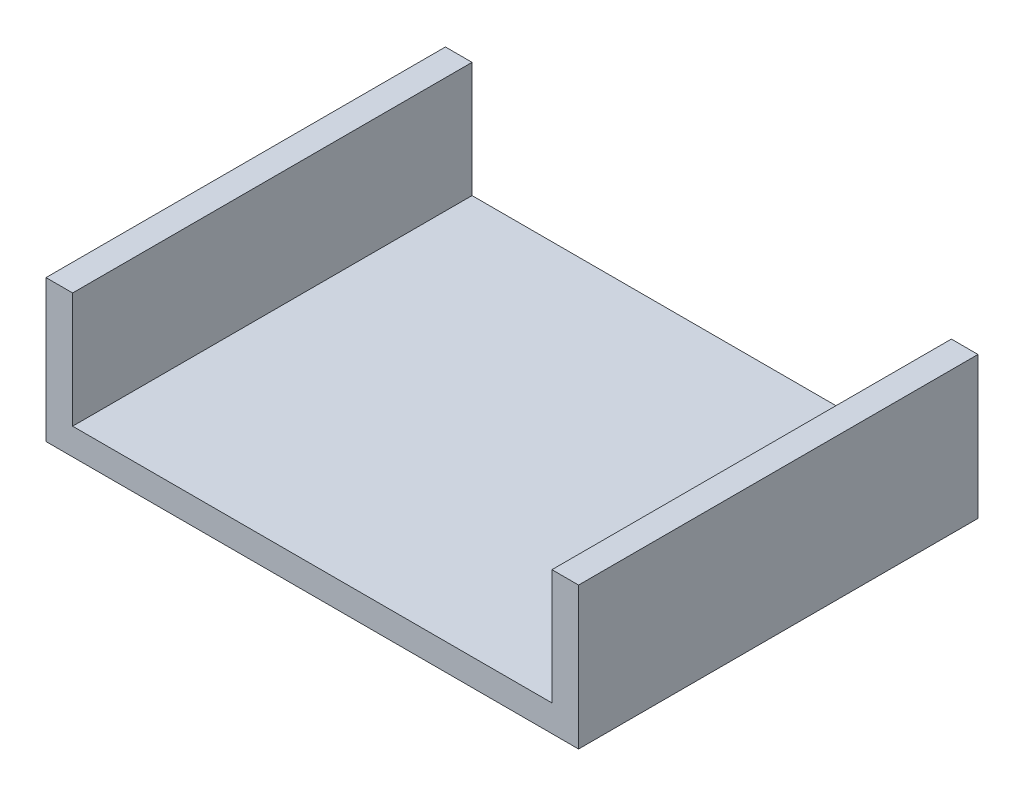
from build123d import *

# Parameters (mm, degrees)
EXTRUDE_1_DEPTH = 45


with BuildPart() as part:
    # 草图1 → 凸台-拉伸1 (new, symmetric)
    with BuildSketch(Plane.XY):
        Polygon((-60, 0), (60, 0), (60, 32), (54, 32), (54, 6), (-54, 6), (-54, 32), (-60, 32), align=None)
    extrude(amount=EXTRUDE_1_DEPTH, both=True)


solid = part.part
